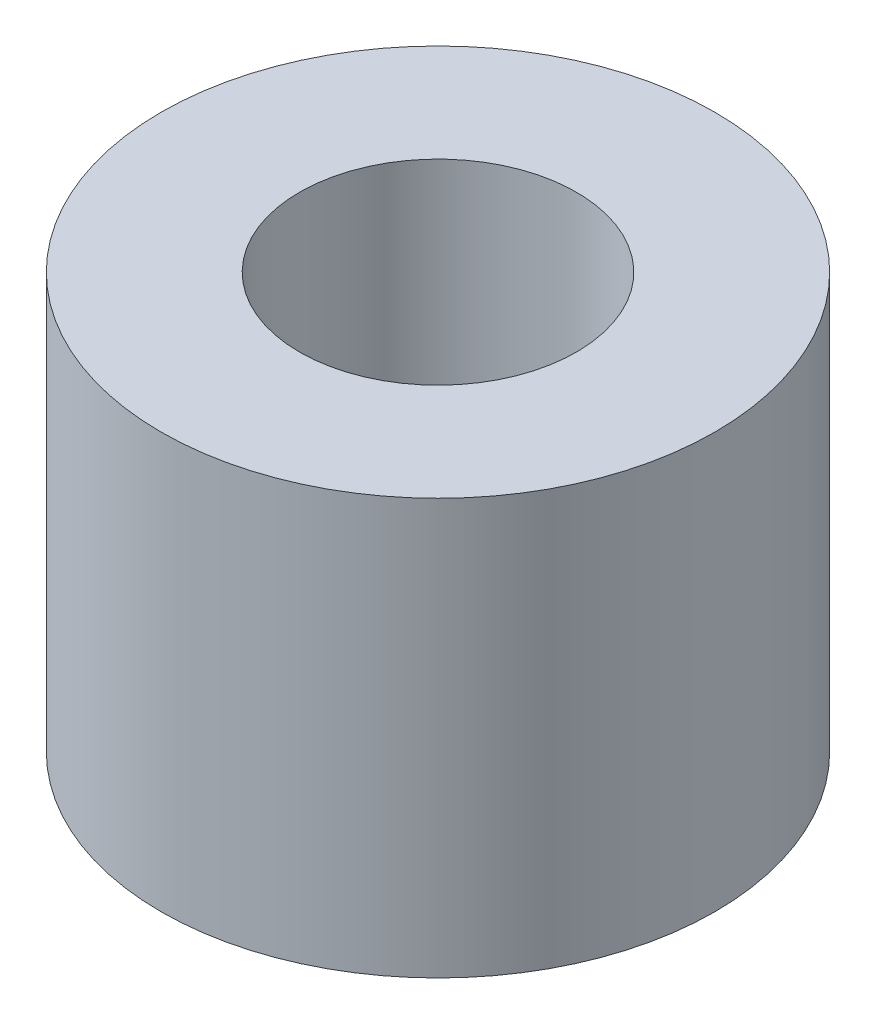
from build123d import *

# Parameters (mm, degrees)
SKETCH1_W = 2
SKETCH1_H = 6


with BuildPart() as part:
    # Sketch1 → Revolve1 (revolve)
    with BuildSketch(Plane.XY, mode=Mode.PRIVATE) as revolve1_sk:
        with Locations((-3, 3)):
            Rectangle(SKETCH1_W, SKETCH1_H)
    revolve(revolve1_sk.sketch.rotate(Axis((0, 8.416352699, 0), (0, -1, 0)), 270), axis=Axis((0, 8.416352699, 0), (0, -1, 0)))


solid = part.part
